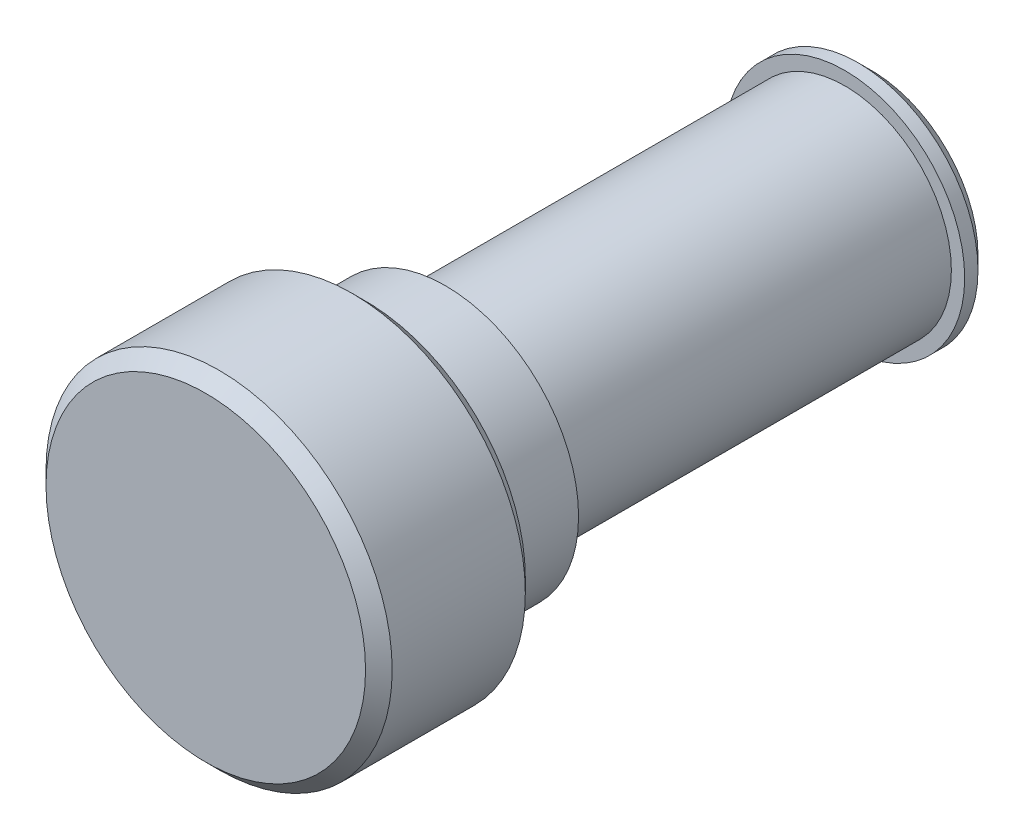
from build123d import *

# Parameters (mm, degrees)
SKETCH1_R           = 4.5
BOSS_EXTRUDE1_DEPTH = 1
SKETCH2_R           = 4
BOSS_EXTRUDE2_DEPTH = 1
SKETCH3_R           = 4
BOSS_EXTRUDE3_DEPTH = 14
SKETCH4_R           = 5
BOSS_EXTRUDE4_DEPTH = 3
SKETCH5_R           = 6.5
BOSS_EXTRUDE5_DEPTH = 6
CHAMFER1_SIZE       = 0.5


with BuildPart() as part:
    # Sketch1 → Boss-Extrude1 (new body)
    with BuildSketch(Plane.XY):
        Circle(SKETCH1_R)
    extrude(amount=BOSS_EXTRUDE1_DEPTH)

    # Sketch2 → Boss-Extrude2 (add)
    with BuildSketch(Plane.XY.offset(1)):
        Circle(SKETCH2_R)
    extrude(amount=BOSS_EXTRUDE2_DEPTH)

    # Sketch3 → Boss-Extrude3 (add)
    with BuildSketch(Plane.XY.offset(2)):
        Circle(SKETCH3_R)
    extrude(amount=BOSS_EXTRUDE3_DEPTH)

    # Sketch4 → Boss-Extrude4 (add)
    with BuildSketch(Plane.XY.offset(16)):
        Circle(SKETCH4_R)
    extrude(amount=BOSS_EXTRUDE4_DEPTH)

    # Sketch5 → Boss-Extrude5 (add)
    with BuildSketch(Plane.XY.offset(19)):
        Circle(SKETCH5_R)
    extrude(amount=BOSS_EXTRUDE5_DEPTH)

    # Chamfer1
    chamfer1_edges = [part.edges().sort_by_distance(p)[0] for p in [
        (-6.5, 0, 19),
        (-6.5, 0, 25),
        (-4.5, 0, 0),
    ]]
    chamfer(chamfer1_edges, length=CHAMFER1_SIZE)


solid = part.part
